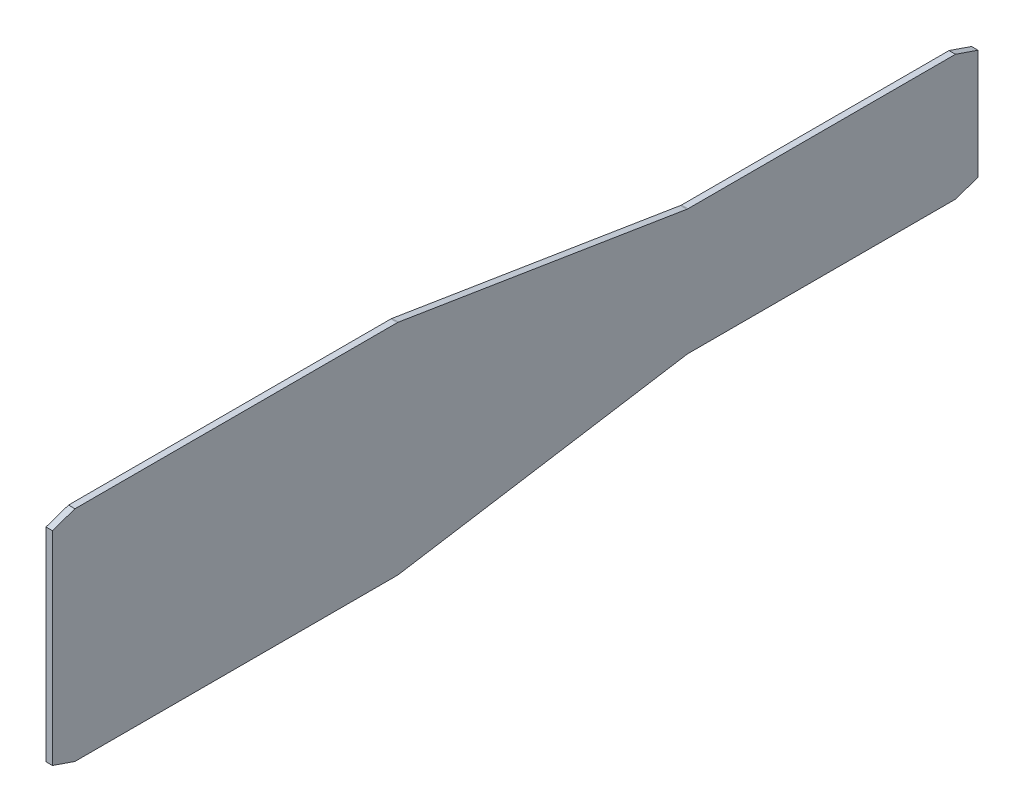
from build123d import *

# Parameters (mm, degrees)
BOSS_EXTRUDE1_DEPTH = 10


with BuildPart() as part:
    # Sketch1 → Boss-Extrude1 (new body)
    with BuildSketch(Plane(origin=(0, 0, 0), x_dir=(0, 0, -1), z_dir=(1, 0, 0))):
        with BuildLine():
            Line((0, -158), (0, 158))
            Line((0, 158), (35, 170))
            Line((35, 170), (535.799605091, 170))
            ThreePointArc((535.799605091, 170), (536.59744846, 169.968121486), (537.390205017, 169.872689192))
            Line((537.390205017, 169.872689192), (985.809794983, 97.627310808))
            ThreePointArc((985.809794983, 97.627310808), (986.60255154, 97.531878514), (987.400394909, 97.5))
            Line((987.400394909, 97.5), (1403, 97.5))
            Line((1403, 97.5), (1438, 85.5))
            Line((1438, 85.5), (1438, -85.5))
            Line((1438, -85.5), (1403, -97.5))
            Line((1403, -97.5), (987.400394909, -97.5))
            ThreePointArc((987.400394909, -97.5), (986.60255154, -97.531878514), (985.809794983, -97.627310808))
            Line((985.809794983, -97.627310808), (537.390205017, -169.872689192))
            ThreePointArc((537.390205017, -169.872689192), (536.59744846, -169.968121486), (535.799605091, -170))
            Line((535.799605091, -170), (35, -170))
            Line((35, -170), (0, -158))
        make_face()
    extrude(amount=BOSS_EXTRUDE1_DEPTH)


solid = part.part
